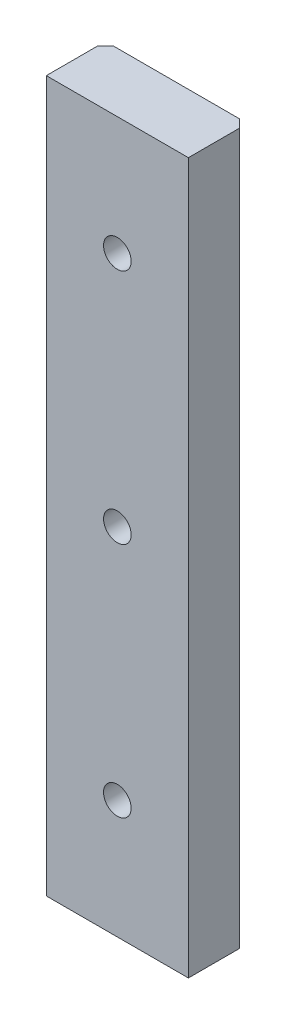
SolidWorks part; units mm, degrees
ref_plane "Front Plane" through (0, 0, 0) normal (0, 0, 1) x (1, 0, 0)
ref_plane "Top Plane" through (0, 0, 0) normal (0, 1, 0) x (1, 0, 0)
ref_plane "Right Plane" through (0, 0, 0) normal (1, 0, 0) x (0, 0, -1)
sketch "Sketch1" plane through (0, 0, 0) normal (0, 1, 0) x (1, 0, 0)
  line L1 (-9, 3.75) -> (9, 3.75)
  line L2 (-9, 3.75) -> (-9, -3.75)
  line L3 (-9, -3.75) -> (9, -3.75)
  line L4 (9, 3.75) -> (9, -3.75)
  line L5 (-9, 3.75) -> (9, -3.75) construction
  line L6 (-9, -3.75) -> (9, 3.75) construction
  point P0 (0, 0)
  dimension "D1" = 18
  dimension "D2" = 7.5
extrude "Boss-Extrude1" add sketch "Sketch1" along normal blind 90
chamfer "Chamfer1" distance 1 angle 45 2 edges at (-9, 45, -3.75) (9, 45, -3.75)
sketch "Sketch2" plane through (0, 0, -3.75) normal (0, 0, -1) x (-1, 0, 0)
  line L0 (0, 0) -> (0, 50000) construction
  line L1 (-8, 0) -> (8, 0) construction
  circle A0 centre (0, 15) radius 1.75
  dimension "D1" = 3.5
  dimension "D2" = 15
extrude "Cut-Extrude1" cut sketch "Sketch2" against normal through all
sketch "Sketch3" plane through (0, 0, -3.75) normal (0, 0, -1) x (-1, 0, 0)
  circle A0 centre (0, 15) radius 3
  dimension "D1" = 6
extrude "Cut-Extrude2" cut sketch "Sketch3" against normal blind 4.5
pattern_linear "LPattern1" count 4 spacing 30 along (0, 1, 0) of "Cut-Extrude2"
pattern_linear "LPattern2" count 4 spacing 30 along (0, 1, 0) of "Cut-Extrude1"
